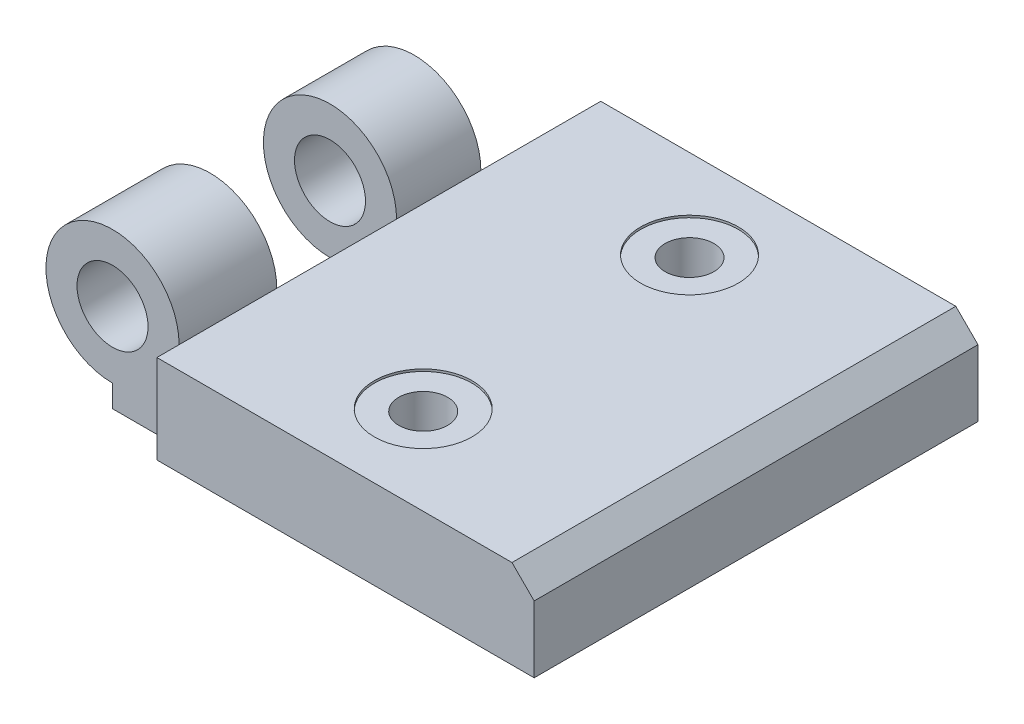
from build123d import *

# Parameters (mm, degrees)
EXTRUDE_2_DEPTH               = 50
CUT_EXTRUDE_1_DEPTH           = 122.86057607
CUT_EXTRUDE_1_DEPTH_BACK      = 122.86057607
SKETCH_2_R                    = 8
CUT_EXTRUDE_8_DEPTH           = 85.409715081
CUT_EXTRUDE_8_DEPTH_BACK      = 85.409715081
SKETCH_3_W                    = 34.567648094
SKETCH_3_H                    = 27
SKETCH_3_W_2                  = 34.56764798
SKETCH_3_H_2                  = 5
CHAMFER_1_SIZE                = 5
HOLE_WIZARD_M10_1_D           = 11
HOLE_WIZARD_M10_1_CBORE_D     = 22
HOLE_WIZARD_M10_1_CBORE_DEPTH = 0.5


with BuildPart() as part:
    # 草图1 → 凸台-拉伸2 (new, symmetric)
    with BuildSketch(Plane.XY):
        with BuildLine():
            Line((-50, -10), (50, -10))
            Line((50, -10), (50, 10))
            Line((50, 10), (-35, 10))
            ThreePointArc((-35, 10), (-60.606601718, 20.606601718), (-50, -5))
            Line((-50, -5), (-50, -10))
        make_face()
    extrude(amount=EXTRUDE_2_DEPTH, both=True)

    # 草图2 → 切除-拉伸1 (cut, two sides: drawn at the far end of the back side and taken through both)
    with BuildSketch(Plane.XY.offset(50).offset(-CUT_EXTRUDE_1_DEPTH_BACK)):
        with Locations((-50, 10)):
            Circle(SKETCH_2_R)
    extrude(amount=CUT_EXTRUDE_1_DEPTH + CUT_EXTRUDE_1_DEPTH_BACK, mode=Mode.SUBTRACT)

    # 草图3 → 切除-拉伸8 (cut, two sides: drawn at the far end of the back side and taken through both)
    with BuildSketch(Plane(origin=(0, 10, 0), x_dir=(1, 0, 0), z_dir=(0, 1, 0)).offset(-CUT_EXTRUDE_8_DEPTH_BACK)):
        Polygon((-69.567648094, 22.997195123), (-35, 22.997195123), (-35, 50), (-69.107419327, 50), align=None)
        with Locations((-52.283824047, -9.502804877)):
            Rectangle(SKETCH_3_W, SKETCH_3_H)
        with Locations((-52.28382399, -47.5)):
            Rectangle(SKETCH_3_W_2, SKETCH_3_H_2)
    extrude(amount=CUT_EXTRUDE_8_DEPTH + CUT_EXTRUDE_8_DEPTH_BACK, mode=Mode.SUBTRACT)

    # 倒角1
    chamfer_1_edges = [part.edges().sort_by_distance(p)[0] for p in [
        (50, 10, 0),
    ]]
    chamfer(chamfer_1_edges, length=CHAMFER_1_SIZE)

    # M10 六角头螺栓的柱形沉头孔1 (through all)
    with Locations(Plane(origin=(5, 10, -30), x_dir=(0, 0, 1), z_dir=(0, 1, 0))):
        with Locations((0, 0)):
            hole_wizard_m10_1 = CounterBoreHole(HOLE_WIZARD_M10_1_D / 2, HOLE_WIZARD_M10_1_CBORE_D / 2, HOLE_WIZARD_M10_1_CBORE_DEPTH)

    # 镜向1: M10 六角头螺栓的柱形沉头孔1 across plane
    add(hole_wizard_m10_1.mirror(Plane.XY), mode=Mode.SUBTRACT)


solid = part.part
